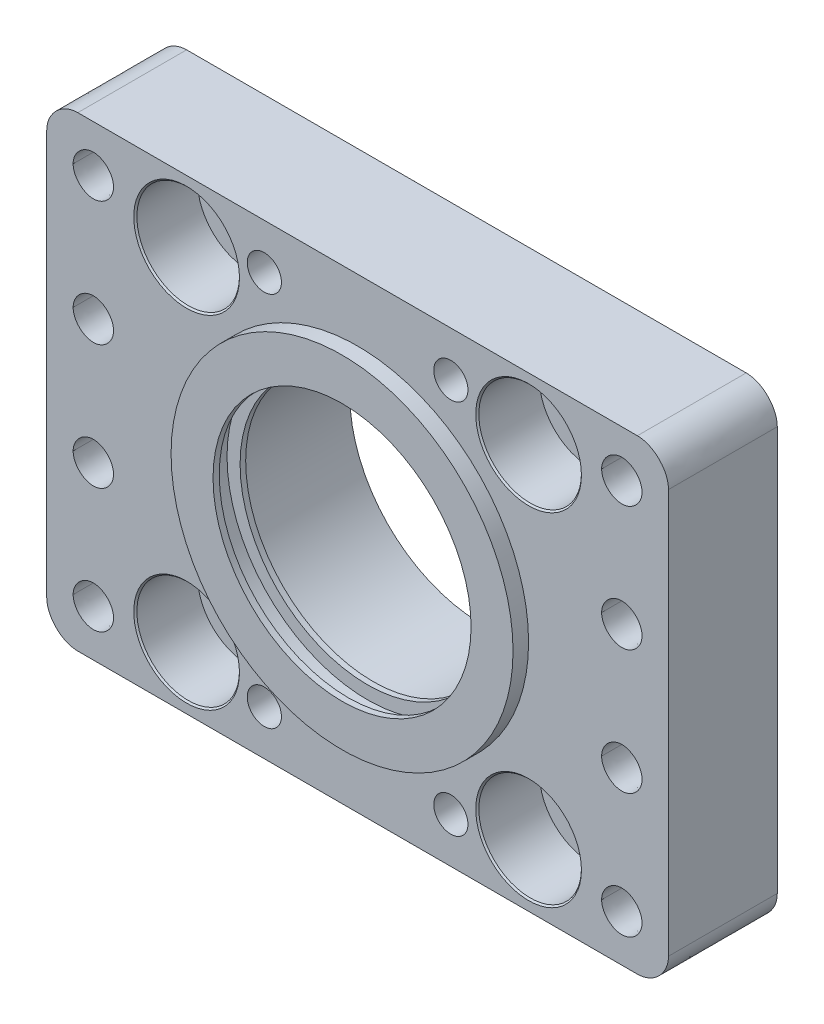
from build123d import *

# Parameters (mm, degrees)
SKETCH2_R           = 8.25
BOSS_EXTRUDE1_DEPTH = 35
SKETCH4_R           = 3.3
CUT_EXTRUDE1_DEPTH  = 35
SKETCH5_R           = 16.5
CUT_EXTRUDE2_DEPTH  = 20
SKETCH6_R           = 5.5
CUT_EXTRUDE3_DEPTH  = 10
SKETCH7_R           = 62.5
BOSS_EXTRUDE2_DEPTH = 5
CHAMFER2_SIZE       = 0.5
SKETCH9_R           = 55
BOSS_EXTRUDE3_DEPTH = 5
SKETCH12_R          = 42.5
CUT_EXTRUDE7_DEPTH  = 35
SKETCH13_R          = 41
CUT_EXTRUDE8_DEPTH  = 35
SKETCH14_R          = 45.2
CUT_EXTRUDE9_DEPTH  = 6.2
SKETCH15_R          = 41.5
CUT_EXTRUDE10_DEPTH = 6.2


with BuildPart() as part:
    # Sketch2 → Boss-Extrude1 (new body)
    with BuildSketch(Plane.XY):
        with BuildLine():
            add(Edge.make_bspline(
                [(-106.250646967, -65), (-106.250646967, -21.666666667), (-106.250646967, 21.666666667), (-106.250646967, 65)],
                knots=[0, 0, 0, 0, 1, 1, 1, 1], degree=3))
            add(Edge.make_bspline(
                [(-106.250646967, 65), (-106.250646967, 70.235987756), (-101.486634723, 75), (-96.250646967, 75)],
                knots=[0, 0, 0, 0, 1, 1, 1, 1], degree=3))
            add(Edge.make_bspline(
                [(83.749353033, 75), (23.749353033, 75), (-36.250646967, 75), (-96.250646967, 75)],
                knots=[0, 0, 0, 0, 1, 1, 1, 1], degree=3))
            add(Edge.make_bspline(
                [(83.749353033, 75), (88.985340789, 75), (93.749353033, 70.235987756), (93.749353033, 65)],
                knots=[0, 0, 0, 0, 1, 1, 1, 1], degree=3))
            add(Edge.make_bspline(
                [(93.749353033, 65), (93.749353033, 21.666666667), (93.749353033, -21.666666667), (93.749353033, -65)],
                knots=[0, 0, 0, 0, 1, 1, 1, 1], degree=3))
            add(Edge.make_bspline(
                [(93.749353033, -65), (93.749353033, -70.235987756), (88.985340789, -75), (83.749353033, -75)],
                knots=[0, 0, 0, 0, 1, 1, 1, 1], degree=3))
            add(Edge.make_bspline(
                [(-96.250646967, -75), (-36.250646967, -75), (23.749353033, -75), (83.749353033, -75)],
                knots=[0, 0, 0, 0, 1, 1, 1, 1], degree=3))
            add(Edge.make_bspline(
                [(-96.250646967, -75), (-101.486634723, -75), (-106.250646967, -70.235987756), (-106.250646967, -65)],
                knots=[0, 0, 0, 0, 1, 1, 1, 1], degree=3))
        make_face()
        with Locations((48.749353033, 55)):
            Circle(SKETCH2_R, mode=Mode.SUBTRACT)
        with BuildLine():
            add(Edge.make_bspline(
                [(-53.000646967, -55), (-53.000646967, -59.330672713), (-56.922862803, -63.24942583), (-65.57843113, -63.25057417), (-69.500646967, -59.33656635), (-69.500646967, -55)],
                knots=[0, 0, 0, 0, 0.5, 0.5, 1, 1, 1, 1], degree=3))
            add(Edge.make_bspline(
                [(-69.500646967, -55), (-69.500646967, -50.669327287), (-65.57843113, -46.75057417), (-56.922862803, -46.74942583), (-53.000646967, -50.663433649), (-53.000646967, -55)],
                knots=[0, 0, 0, 0, 0.5, 0.5, 1, 1, 1, 1], degree=3))
        make_face(mode=Mode.SUBTRACT)
        with BuildLine():
            add(Edge.make_bspline(
                [(56.999353033, -55), (56.999353033, -59.330672713), (53.077137197, -63.24942583), (44.42156887, -63.25057417), (40.499353033, -59.336566351), (40.499353033, -55)],
                knots=[0, 0, 0, 0, 0.5, 0.5, 1, 1, 1, 1], degree=3))
            add(Edge.make_bspline(
                [(40.499353033, -55), (40.499353033, -50.669327287), (44.42156887, -46.75057417), (53.077137197, -46.74942583), (56.999353033, -50.663433649), (56.999353033, -55)],
                knots=[0, 0, 0, 0, 0.5, 0.5, 1, 1, 1, 1], degree=3))
        make_face(mode=Mode.SUBTRACT)
        with BuildLine():
            add(Edge.make_bspline(
                [(-53.000646967, 55), (-53.000646967, 50.669327287), (-56.922862803, 46.75057417), (-65.57843113, 46.74942583), (-69.500646967, 50.663433649), (-69.500646967, 55)],
                knots=[0, 0, 0, 0, 0.5, 0.5, 1, 1, 1, 1], degree=3))
            add(Edge.make_bspline(
                [(-69.500646967, 55), (-69.500646967, 59.330672713), (-65.57843113, 63.24942583), (-56.922862803, 63.25057417), (-53.000646967, 59.336566351), (-53.000646967, 55)],
                knots=[0, 0, 0, 0, 0.5, 0.5, 1, 1, 1, 1], degree=3))
        make_face(mode=Mode.SUBTRACT)
        with BuildLine():
            add(Edge.make_bspline(
                [(-84.750646967, -60), (-84.750646967, -63.411434987), (-87.842824497, -66.499426175), (-94.658469436, -66.500573825), (-97.750646967, -63.417296748), (-97.750646967, -60)],
                knots=[0, 0, 0, 0, 0.5, 0.5, 1, 1, 1, 1], degree=3))
            add(Edge.make_bspline(
                [(-97.750646967, -60), (-97.750646967, -56.588565013), (-94.658469435, -53.500573825), (-87.842824498, -53.499426175), (-84.750646967, -56.582703252), (-84.750646967, -60)],
                knots=[0, 0, 0, 0, 0.5, 0.5, 1, 1, 1, 1], degree=3))
        make_face(mode=Mode.SUBTRACT)
        with BuildLine():
            add(Edge.make_bspline(
                [(-84.750646967, -20), (-84.750646967, -23.411434987), (-87.842824498, -26.499426175), (-94.658469435, -26.500573825), (-97.750646967, -23.417296748), (-97.750646967, -20)],
                knots=[0, 0, 0, 0, 0.5, 0.5, 1, 1, 1, 1], degree=3))
            add(Edge.make_bspline(
                [(-97.750646967, -20), (-97.750646967, -16.588565013), (-94.658469436, -13.500573825), (-87.842824498, -13.499426175), (-84.750646967, -16.582703252), (-84.750646967, -20)],
                knots=[0, 0, 0, 0, 0.5, 0.5, 1, 1, 1, 1], degree=3))
        make_face(mode=Mode.SUBTRACT)
        with BuildLine():
            add(Edge.make_bspline(
                [(-84.750646967, 20), (-84.750646967, 16.588565013), (-87.842824498, 13.500573825), (-94.658469435, 13.499426175), (-97.750646967, 16.582703252), (-97.750646967, 20)],
                knots=[0, 0, 0, 0, 0.5, 0.5, 1, 1, 1, 1], degree=3))
            add(Edge.make_bspline(
                [(-97.750646967, 20), (-97.750646967, 23.411434987), (-94.658469435, 26.499426175), (-87.842824498, 26.500573825), (-84.750646967, 23.417296749), (-84.750646967, 20)],
                knots=[0, 0, 0, 0, 0.5, 0.5, 1, 1, 1, 1], degree=3))
        make_face(mode=Mode.SUBTRACT)
        with BuildLine():
            add(Edge.make_bspline(
                [(-84.750646967, 60), (-84.750646967, 56.588565013), (-87.842824498, 53.500573825), (-94.658469435, 53.499426175), (-97.750646967, 56.582703252), (-97.750646967, 60)],
                knots=[0, 0, 0, 0, 0.5, 0.5, 1, 1, 1, 1], degree=3))
            add(Edge.make_bspline(
                [(-97.750646967, 60), (-97.750646967, 63.411434987), (-94.658469435, 66.499426175), (-87.842824498, 66.500573825), (-84.750646967, 63.417296748), (-84.750646967, 60)],
                knots=[0, 0, 0, 0, 0.5, 0.5, 1, 1, 1, 1], degree=3))
        make_face(mode=Mode.SUBTRACT)
        with BuildLine():
            add(Edge.make_bspline(
                [(85.249353033, -60), (85.249353033, -63.411434987), (82.157175502, -66.499426175), (75.341530565, -66.500573825), (72.249353033, -63.417296748), (72.249353033, -60)],
                knots=[0, 0, 0, 0, 0.5, 0.5, 1, 1, 1, 1], degree=3))
            add(Edge.make_bspline(
                [(72.249353033, -60), (72.249353033, -56.588565013), (75.341530565, -53.500573825), (82.157175502, -53.499426175), (85.249353033, -56.582703252), (85.249353033, -60)],
                knots=[0, 0, 0, 0, 0.5, 0.5, 1, 1, 1, 1], degree=3))
        make_face(mode=Mode.SUBTRACT)
        with BuildLine():
            add(Edge.make_bspline(
                [(85.249353033, -20), (85.249353033, -23.411434987), (82.157175502, -26.499426175), (75.341530565, -26.500573825), (72.249353033, -23.417296748), (72.249353033, -20)],
                knots=[0, 0, 0, 0, 0.5, 0.5, 1, 1, 1, 1], degree=3))
            add(Edge.make_bspline(
                [(72.249353033, -20), (72.249353033, -16.588565013), (75.341530565, -13.500573825), (82.157175502, -13.499426175), (85.249353033, -16.582703252), (85.249353033, -20)],
                knots=[0, 0, 0, 0, 0.5, 0.5, 1, 1, 1, 1], degree=3))
        make_face(mode=Mode.SUBTRACT)
        with BuildLine():
            add(Edge.make_bspline(
                [(85.249353033, 20), (85.249353033, 16.588565013), (82.157175502, 13.500573825), (75.341530565, 13.499426175), (72.249353033, 16.582703252), (72.249353033, 20)],
                knots=[0, 0, 0, 0, 0.5, 0.5, 1, 1, 1, 1], degree=3))
            add(Edge.make_bspline(
                [(72.249353033, 20), (72.249353033, 23.411434987), (75.341530564, 26.499426175), (82.157175502, 26.500573825), (85.249353033, 23.417296748), (85.249353033, 20)],
                knots=[0, 0, 0, 0, 0.5, 0.5, 1, 1, 1, 1], degree=3))
        make_face(mode=Mode.SUBTRACT)
        with BuildLine():
            add(Edge.make_bspline(
                [(85.249353033, 60), (85.249353033, 56.588565013), (82.157175502, 53.500573825), (75.341530564, 53.499426175), (72.249353033, 56.582703252), (72.249353033, 60)],
                knots=[0, 0, 0, 0, 0.5, 0.5, 1, 1, 1, 1], degree=3))
            add(Edge.make_bspline(
                [(72.249353033, 60), (72.249353033, 63.411434987), (75.341530565, 66.499426175), (82.157175502, 66.500573825), (85.249353033, 63.417296748), (85.249353033, 60)],
                knots=[0, 0, 0, 0, 0.5, 0.5, 1, 1, 1, 1], degree=3))
        make_face(mode=Mode.SUBTRACT)
    extrude(amount=BOSS_EXTRUDE1_DEPTH)

    # Sketch4 → Cut-Extrude1 (cut)
    with BuildSketch(Plane.XY.offset(35)):
        with Locations((-36.250646967, 60.5)):
            Circle(SKETCH4_R)
        with Locations((23.749353033, 60.5)):
            Circle(SKETCH4_R)
        with Locations((23.749353033, -60.5)):
            Circle(SKETCH4_R)
        with Locations((-36.250646967, -60.5)):
            Circle(SKETCH4_R)
    extrude(amount=-CUT_EXTRUDE1_DEPTH, mode=Mode.SUBTRACT)

    # Sketch5 → Cut-Extrude2 (cut)
    with BuildSketch(Plane.XY.offset(35)):
        with Locations((-61.250646967, 55)):
            Circle(SKETCH5_R)
        with Locations((48.749353033, 55)):
            Circle(SKETCH5_R)
        with Locations((48.749353033, -55)):
            Circle(SKETCH5_R)
        with Locations((-61.250646967, -55)):
            Circle(SKETCH5_R)
    extrude(amount=-CUT_EXTRUDE2_DEPTH, mode=Mode.SUBTRACT)

    # Sketch6 → Cut-Extrude3 (cut)
    with BuildSketch(Plane.XY.offset(35)):
        with Locations((-36.250646967, 60.5)):
            Circle(SKETCH6_R)
        with Locations((23.749353033, 60.5)):
            Circle(SKETCH6_R)
        with Locations((23.749353033, -60.5)):
            Circle(SKETCH6_R)
        with Locations((-36.250646967, -60.5)):
            Circle(SKETCH6_R)
    extrude(amount=-CUT_EXTRUDE3_DEPTH, mode=Mode.SUBTRACT)

    # Sketch7 → Boss-Extrude2 (add)
    with BuildSketch(Plane(origin=(0, 0, 0), x_dir=(-1, 0, 0), z_dir=(0, 0, -1))):
        with Locations(Location((6.250646967, 0, 0), (0, 0, 180))):
            Circle(SKETCH7_R)
    extrude(amount=BOSS_EXTRUDE2_DEPTH)

    # Chamfer2
    chamfer2_edges = [part.edges().sort_by_distance(p)[0] for p in [
        (-77.750646967, 55, 35),
        (-77.750646967, -55, 35),
        (32.249353033, -55, 35),
        (32.249353033, 55, 35),
    ]]
    chamfer(chamfer2_edges, length=CHAMFER2_SIZE)

    # Sketch9 → Boss-Extrude3 (add)
    with BuildSketch(Plane.XY.offset(35)):
        with Locations((-6.250646967, 0)):
            Circle(SKETCH9_R)
    extrude(amount=BOSS_EXTRUDE3_DEPTH)

    # Sketch12 → Cut-Extrude7 (cut)
    with BuildSketch(Plane(origin=(0, 0, -5), x_dir=(-1, 0, 0), z_dir=(0, 0, -1))):
        with Locations((6.250646967, 0)):
            Circle(SKETCH12_R)
    extrude(amount=-CUT_EXTRUDE7_DEPTH, mode=Mode.SUBTRACT)

    # Sketch13 → Cut-Extrude8 (cut)
    with BuildSketch(Plane(origin=(0, 0, 30), x_dir=(-1, 0, 0), z_dir=(0, 0, -1))):
        with Locations((6.250646967, 0)):
            Circle(SKETCH13_R)
    extrude(amount=-CUT_EXTRUDE8_DEPTH, mode=Mode.SUBTRACT)

    # Sketch14 → Cut-Extrude9 (cut)
    with BuildSketch(Plane(origin=(0, 0, 31.8), x_dir=(-1, 0, 0), z_dir=(0, 0, -1))):
        with Locations((6.250646967, 0)):
            Circle(SKETCH14_R)
    extrude(amount=-CUT_EXTRUDE9_DEPTH, mode=Mode.SUBTRACT)

    # Sketch15 → Cut-Extrude10 (cut)
    with BuildSketch(Plane(origin=(0, 0, 38), x_dir=(-1, 0, 0), z_dir=(0, 0, -1))):
        with Locations((6.250646967, 0)):
            Circle(SKETCH15_R)
    extrude(amount=-CUT_EXTRUDE10_DEPTH, mode=Mode.SUBTRACT)


solid = part.part
